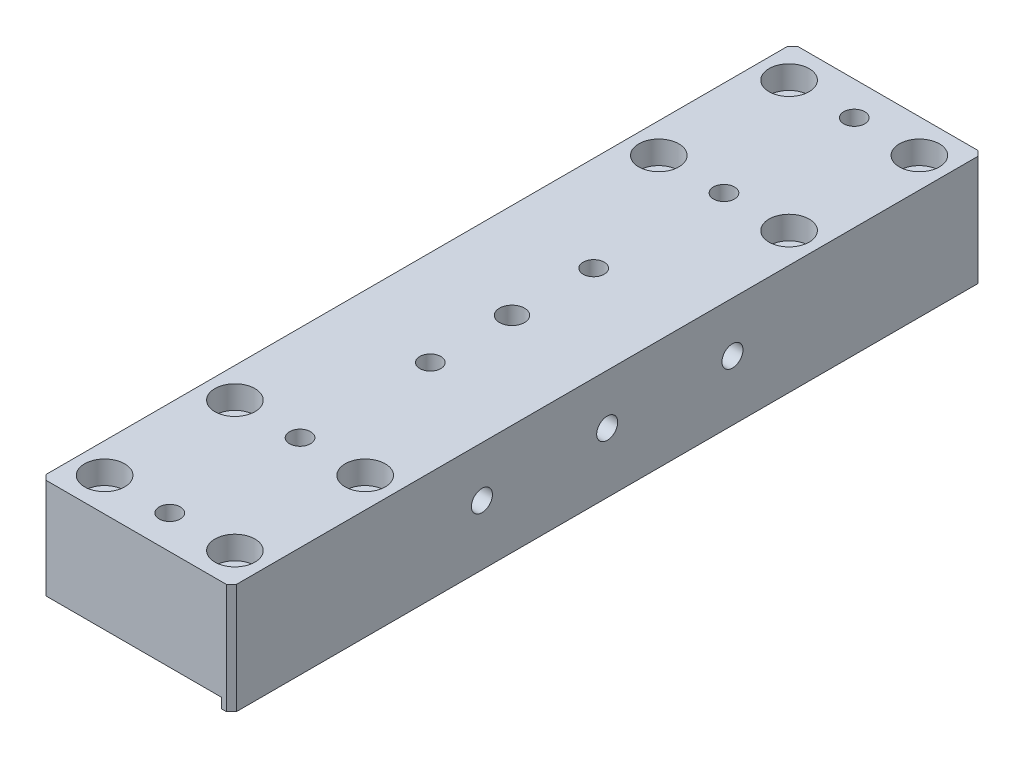
from build123d import *

# Parameters (mm, degrees)
BOSS_EXTRUDE1_DEPTH                                = 75
HOLE_SIZE_SOCKET_HEAD_CAP_SCREW_TYPE_1_D           = 4.5
HOLE_SIZE_SOCKET_HEAD_CAP_SCREW_TYPE_1_CBORE_D     = 8
HOLE_SIZE_SOCKET_HEAD_CAP_SCREW_TYPE_1_CBORE_DEPTH = 4.6
M5_TAPPED_HOLE1_D                                  = 4.2
M5_TAPPED_HOLE1_DEPTH                              = 12.4
M5_TAPPED_HOLE1_TIP                                = 1.2618073
M5_TAPPED_HOLE2_D                                  = 4.2
M5_TAPPED_HOLE2_DEPTH                              = 12.4
M5_TAPPED_HOLE2_TIP                                = 1.2618073
CHAMFER1_SIZE                                      = 1
DOWEL_HOLE1_D                                      = 5
DOWEL_HOLE1_DEPTH                                  = 7.5
DOWEL_HOLE1_TIP                                    = 1.502151548


with BuildPart() as part:
    # Sketch1 → Boss-Extrude1 (new, symmetric)
    with BuildSketch(Plane.XY):
        Polygon((0, 0), (0, 22), (-38, 22), (-38, 2), (-2, 2), (-2, 0), align=None)
    extrude(amount=BOSS_EXTRUDE1_DEPTH, both=True)

    # Hole size (socket head cap screw type)1 (through all)
    with Locations(Plane(origin=(0, 22, 0), x_dir=(1, 0, 0), z_dir=(0, 1, 0))):
        with Locations((-32, -68.3), (-32, 68.3), (-6, 42.3), (-32, 42.3), (-6, 68.3), (-6, -68.3), (-6, -42.3), (-32, -42.3)):
            CounterBoreHole(HOLE_SIZE_SOCKET_HEAD_CAP_SCREW_TYPE_1_D / 2, HOLE_SIZE_SOCKET_HEAD_CAP_SCREW_TYPE_1_CBORE_D / 2, HOLE_SIZE_SOCKET_HEAD_CAP_SCREW_TYPE_1_CBORE_DEPTH)

    # M5 Tapped Hole1
    with Locations(Plane(origin=(0, 0, 0), x_dir=(0, 0, -1), z_dir=(1, 0, 0))):
        with Locations((0, 12), (-25, 12), (25, 12)):
            Hole(M5_TAPPED_HOLE1_D / 2, depth=M5_TAPPED_HOLE1_DEPTH)
            with Locations((0, 0, -(M5_TAPPED_HOLE1_DEPTH + M5_TAPPED_HOLE1_TIP / 2))):  # 118° drill point
                Cone(0, M5_TAPPED_HOLE1_D / 2, M5_TAPPED_HOLE1_TIP, mode=Mode.SUBTRACT)

    # M5 Tapped Hole2
    with Locations(Plane(origin=(0, 22, 0), x_dir=(1, 0, 0), z_dir=(0, 1, 0))):
        with Locations((-19, -16.3), (-19, 68.3), (-19, 42.3), (-19, -42.3), (-19, -68.3), (-19, 16.3)):
            Hole(M5_TAPPED_HOLE2_D / 2, depth=M5_TAPPED_HOLE2_DEPTH)
            with Locations((0, 0, -(M5_TAPPED_HOLE2_DEPTH + M5_TAPPED_HOLE2_TIP / 2))):  # 118° drill point
                Cone(0, M5_TAPPED_HOLE2_D / 2, M5_TAPPED_HOLE2_TIP, mode=Mode.SUBTRACT)

    # Chamfer1
    chamfer1_edges = [part.edges().sort_by_distance(p)[0] for p in [
        (-38, 12, 75),
        (-38, 12, -75),
        (0, 11, -75),
        (0, 11, 75),
    ]]
    chamfer(chamfer1_edges, length=CHAMFER1_SIZE)

    # Dowel Hole1
    with Locations(Plane(origin=(0, 22, 0), x_dir=(1, 0, 0), z_dir=(0, 1, 0))):
        with Locations((-19, 0)):
            Hole(DOWEL_HOLE1_D / 2, depth=DOWEL_HOLE1_DEPTH)
            with Locations((0, 0, -(DOWEL_HOLE1_DEPTH + DOWEL_HOLE1_TIP / 2))):  # 118° drill point
                Cone(0, DOWEL_HOLE1_D / 2, DOWEL_HOLE1_TIP, mode=Mode.SUBTRACT)


solid = part.part
